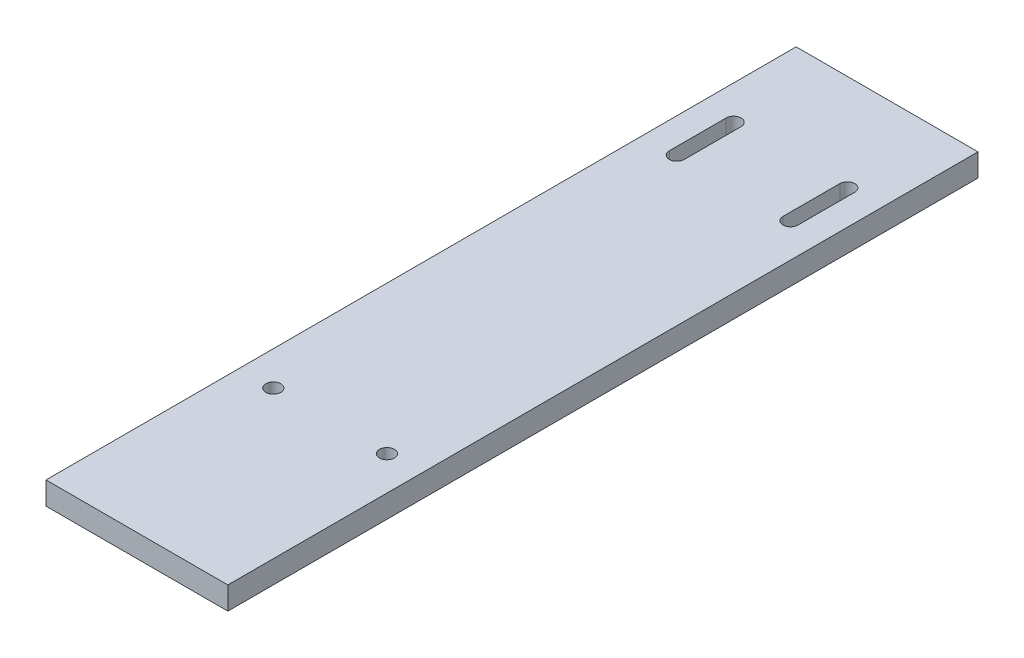
from build123d import *

# Parameters (mm, degrees)
SKETCH1_W                  = 80
SKETCH1_H                  = 330
BOSS_EXTRUDE1_DEPTH        = 10
F_6_6_6_6_DIAMETER_HOLE1_D = 6.6
CUT_EXTRUDE1_DEPTH         = 10


with BuildPart() as part:
    # Sketch1 → Boss-Extrude1 (new body)
    with BuildSketch(Plane(origin=(0, 0, 0), x_dir=(1, 0, 0), z_dir=(0, 1, 0))):
        Rectangle(SKETCH1_W, SKETCH1_H)
    extrude(amount=BOSS_EXTRUDE1_DEPTH)

    # Ø6.6 (6.6) Diameter Hole1 (through all)
    with Locations(Plane(origin=(0, 10, 0), x_dir=(1, 0, 0), z_dir=(0, 1, 0))):
        with Locations((-25, -80), (25, -80)):
            Hole(F_6_6_6_6_DIAMETER_HOLE1_D / 2)

    # Sketch5 → Cut-Extrude1 (cut)
    with BuildSketch(Plane(origin=(0, 10, 0), x_dir=(1, 0, 0), z_dir=(0, 1, 0))):
        with BuildLine():
            Line((-28.3, 97.5), (-28.3, 122.5))
            ThreePointArc((-28.3, 122.5), (-25, 125.8), (-21.7, 122.5))
            Line((-21.7, 122.5), (-21.7, 97.5))
            ThreePointArc((-21.7, 97.5), (-25, 94.2), (-28.3, 97.5))
        make_face()
        with BuildLine():
            Line((21.7, 97.5), (21.7, 122.5))
            ThreePointArc((21.7, 122.5), (25, 125.8), (28.3, 122.5))
            Line((28.3, 122.5), (28.3, 97.5))
            ThreePointArc((28.3, 97.5), (25, 94.2), (21.7, 97.5))
        make_face()
    extrude(amount=-CUT_EXTRUDE1_DEPTH, mode=Mode.SUBTRACT)


solid = part.part
